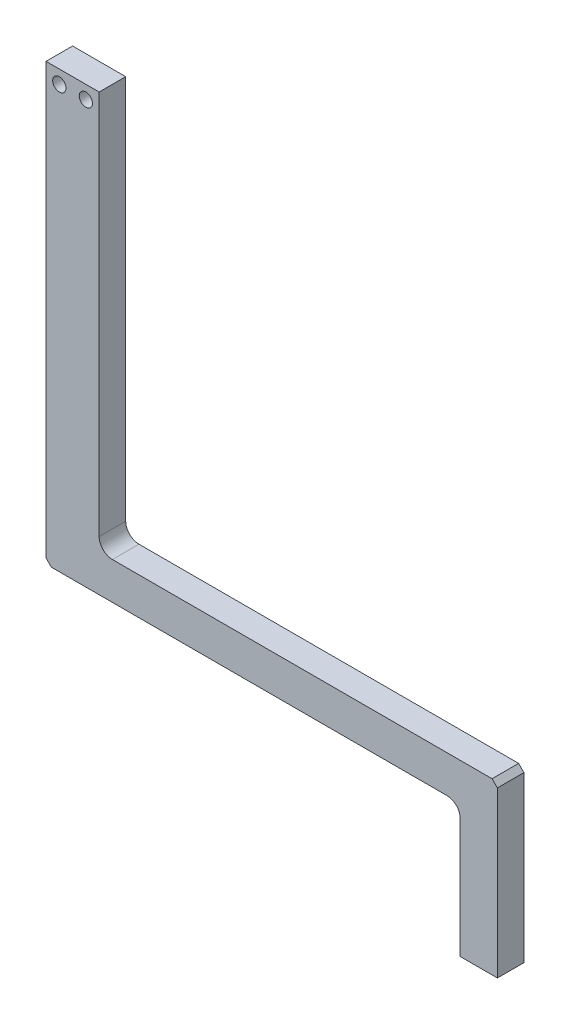
from build123d import *

# Parameters (mm, degrees)
EXTRUDE_1_DEPTH     = 5
CUT_EXTRUDE_1_REACH = 186.989
SKETCH_2_R          = 2.5
SKETCH_3_W          = 14
SKETCH_3_H          = 50
EXTRUDE_2_DEPTH     = 10
FILLET_1_R          = 5
CHAMFER_1_SIZE      = 2


with BuildPart() as part:
    # 草图1 → 凸台-拉伸1 (new, symmetric)
    with BuildSketch(Plane.XY):
        Polygon((0, 0), (-85, 0), (-85, 164), (-65, 164), (-65, 14), (85, 14), (85, 0), align=None)
    extrude(amount=EXTRUDE_1_DEPTH, both=True)

    # 草图2 → 切除-拉伸1 (cut, up to next)
    with BuildSketch(Plane.XY.offset(5), mode=Mode.PRIVATE) as cut_extrude_1_sk1:
        with Locations((-80, 159)):
            Circle(SKETCH_2_R)
    cut_extrude_1_tool1 = extrude(cut_extrude_1_sk1.sketch, amount=-CUT_EXTRUDE_1_REACH, mode=Mode.PRIVATE) & part.part
    # 草图2 → 切除-拉伸1 (cut, up to next)
    with BuildSketch(Plane.XY.offset(5), mode=Mode.PRIVATE) as cut_extrude_1_sk2:
        with Locations((-70, 159)):
            Circle(SKETCH_2_R)
    cut_extrude_1_tool2 = extrude(cut_extrude_1_sk2.sketch, amount=-CUT_EXTRUDE_1_REACH, mode=Mode.PRIVATE) & part.part
    add(cut_extrude_1_tool1.solids().sort_by_distance((-80, 159, 5))[0], mode=Mode.SUBTRACT)
    add(cut_extrude_1_tool2.solids().sort_by_distance((-70, 159, 5))[0], mode=Mode.SUBTRACT)

    # 草图3 → 凸台-拉伸2 (add)
    with BuildSketch(Plane.XY.offset(5)):
        with Locations((78, -25)):
            Rectangle(SKETCH_3_W, SKETCH_3_H)
    extrude(amount=-EXTRUDE_2_DEPTH)

    # 圆角1
    fillet_1_edges = [part.edges().sort_by_distance(p)[0] for p in [
        (-65, 14, 0),
        (71, 0, 0),
    ]]
    fillet(fillet_1_edges, radius=FILLET_1_R)

    # 倒角1
    chamfer_1_edges = [part.edges().sort_by_distance(p)[0] for p in [
        (-85, 0, 0),
        (85, 14, 0),
    ]]
    chamfer(chamfer_1_edges, length=CHAMFER_1_SIZE)


solid = part.part
